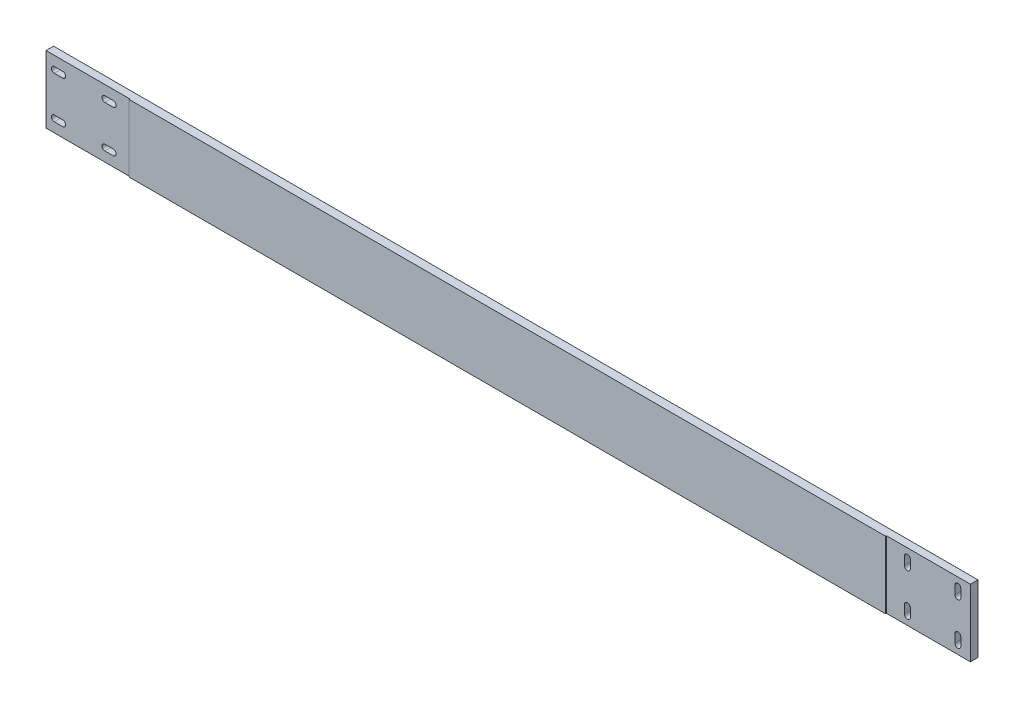
from build123d import *

# Parameters (mm, degrees)
SKETCH_1_W             = 1100
SKETCH_1_H             = 80
EXTRUDE_1_DEPTH        = 10
SKETCH_2_W             = 100
SKETCH_2_H             = 80
CUT_EXTRUDE_1_DEPTH    = 1
HOLE_WIZARD_M6_1_D     = 7
HOLE_WIZARD_M6_1_DEPTH = 22.25
HOLE_WIZARD_M6_1_TIP   = 2.103012167
CUT_EXTRUDE_2_DEPTH    = 552.543289326


with BuildPart() as part:
    # 草图1 → 凸台-拉伸1 (new body)
    with BuildSketch(Plane.XY):
        Rectangle(SKETCH_1_W, SKETCH_1_H)
    extrude(amount=EXTRUDE_1_DEPTH)

    # 草图2 → 切除-拉伸1 (cut)
    with BuildSketch(Plane.XY.offset(10)):
        with Locations((-500, 0)):
            Rectangle(SKETCH_2_W, SKETCH_2_H)
        with Locations((500, 0)):
            Rectangle(SKETCH_2_W, SKETCH_2_H)
    extrude(amount=-CUT_EXTRUDE_1_DEPTH, mode=Mode.SUBTRACT)

    # M6 间隙孔1
    with Locations(Plane(origin=(0, 0, 0), x_dir=(-1, 0, 0), z_dir=(0, 0, -1))):
        with Locations((-535, 25), (475, -25), (535, 25), (535, -25), (475, 25), (-475, 25), (-475, -25), (-535, -25)):
            Hole(HOLE_WIZARD_M6_1_D / 2, depth=HOLE_WIZARD_M6_1_DEPTH)
            with Locations((0, 0, -(HOLE_WIZARD_M6_1_DEPTH + HOLE_WIZARD_M6_1_TIP / 2))):  # 118° drill point
                Cone(0, HOLE_WIZARD_M6_1_D / 2, HOLE_WIZARD_M6_1_TIP, mode=Mode.SUBTRACT)

    # 草图5 → 切除-拉伸2 (cut, through all)
    with BuildSketch(Plane(origin=(0, 0, 0), x_dir=(-1, 0, 0), z_dir=(0, 0, -1))):
        with BuildLine():
            Line((470, 28.5), (480, 28.5))
            ThreePointArc((480, 28.5), (483.5, 25), (480, 21.5))
            Line((480, 21.5), (470, 21.5))
            ThreePointArc((470, 21.5), (466.5, 25), (470, 28.5))
        make_face()
        with BuildLine():
            Line((530, 28.5), (540, 28.5))
            ThreePointArc((540, 28.5), (543.5, 25), (540, 21.5))
            Line((540, 21.5), (530, 21.5))
            ThreePointArc((530, 21.5), (526.5, 25), (530, 28.5))
        make_face()
        with BuildLine():
            Line((530, -21.5), (540, -21.5))
            ThreePointArc((540, -21.5), (543.5, -25), (540, -28.5))
            Line((540, -28.5), (530, -28.5))
            ThreePointArc((530, -28.5), (526.5, -25), (530, -21.5))
        make_face()
        with BuildLine():
            Line((470, -21.5), (480, -21.5))
            ThreePointArc((480, -21.5), (483.5, -25), (480, -28.5))
            Line((480, -28.5), (470, -28.5))
            ThreePointArc((470, -28.5), (466.5, -25), (470, -21.5))
        make_face()
        with BuildLine():
            Line((-531.5, 30), (-531.5, 20))
            ThreePointArc((-531.5, 20), (-535, 16.5), (-538.5, 20))
            Line((-538.5, 20), (-538.5, 30))
            ThreePointArc((-538.5, 30), (-535, 33.5), (-531.5, 30))
        make_face()
        with BuildLine():
            Line((-471.5, 30), (-471.5, 20))
            ThreePointArc((-471.5, 20), (-475, 16.5), (-478.5, 20))
            Line((-478.5, 20), (-478.5, 30))
            ThreePointArc((-478.5, 30), (-475, 33.5), (-471.5, 30))
        make_face()
        with BuildLine():
            Line((-538.5, -30), (-538.5, -20))
            ThreePointArc((-538.5, -20), (-535, -16.5), (-531.5, -20))
            Line((-531.5, -20), (-531.5, -30))
            ThreePointArc((-531.5, -30), (-535, -33.5), (-538.5, -30))
        make_face()
        with BuildLine():
            Line((-478.5, -30), (-478.5, -20))
            ThreePointArc((-478.5, -20), (-475, -16.5), (-471.5, -20))
            Line((-471.5, -20), (-471.5, -30))
            ThreePointArc((-471.5, -30), (-475, -33.5), (-478.5, -30))
        make_face()
    extrude(amount=-CUT_EXTRUDE_2_DEPTH, mode=Mode.SUBTRACT)


solid = part.part
